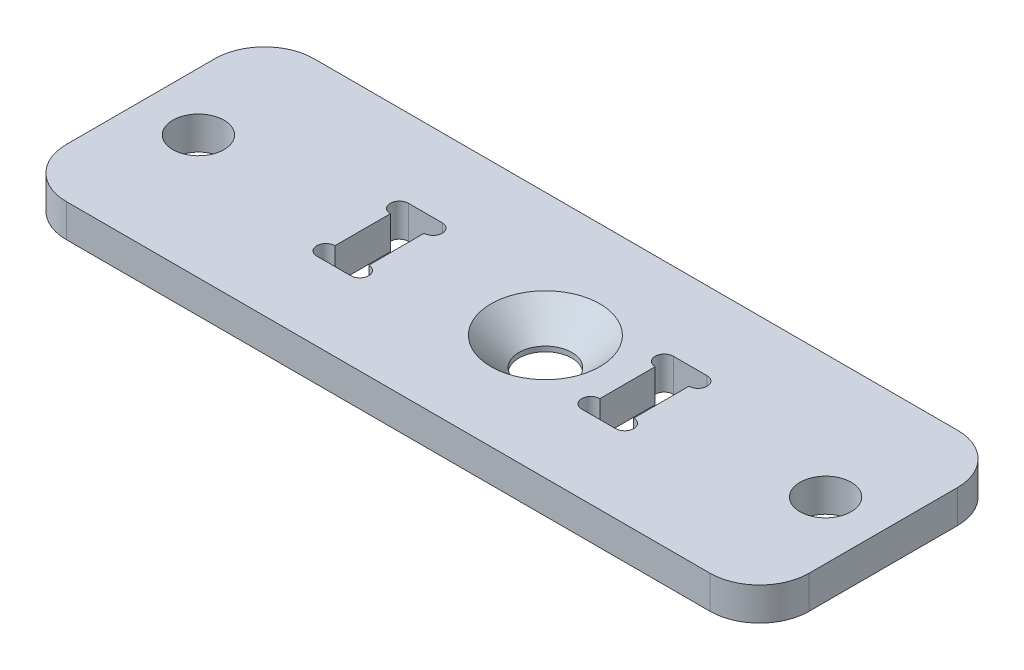
SolidWorks part; units mm, degrees
material "Thornel Mat VMA"
ref_plane "前视基准面" through (0, 0, 0) normal (0, 0, 1) x (1, 0, 0)
ref_plane "上视基准面" through (0, 0, 0) normal (0, 1, 0) x (1, 0, 0)
ref_plane "右视基准面" through (0, 0, 0) normal (1, 0, 0) x (0, 0, -1)
other "Configuration Table"
sketch "草图1" plane through (0, 0, 0) normal (0, 1, 0) x (1, 0, 0)
  line L0 (0, 0) -> (37.6995, 0) construction
  line L1 (-22.5, 7.5) -> (22.5, 7.5)
  line L2 (-22.5, 7.5) -> (-22.5, -7.5)
  line L3 (-22.5, -7.5) -> (22.5, -7.5)
  line L4 (22.5, 7.5) -> (22.5, -7.5)
  line L5 (-22.5, 7.5) -> (22.5, -7.5) construction
  line L6 (-22.5, -7.5) -> (22.5, 7.5) construction
  line L7 (0, 0) -> (0, 17.3296) construction
  line L8 (8.025, 0) -> (8.025, 5.6188) construction
  line L9 (7, 2.775) -> (9.05, 2.775)
  line L10 (7, 2.775) -> (7, -2.775)
  line L11 (7, -2.775) -> (9.05, -2.775)
  line L12 (9.05, 2.775) -> (9.05, -2.775)
  line L13 (7, 2.775) -> (9.05, -2.775) construction
  line L14 (7, -2.775) -> (9.05, 2.775) construction
  line L15 (-7, -2.775) -> (-9.05, 2.775) construction
  line L16 (-7, 2.775) -> (-9.05, -2.775) construction
  line L21 (-9.05, 2.775) -> (-9.05, -2.775)
  line L22 (-7, -2.775) -> (-9.05, -2.775)
  line L23 (-7, 2.775) -> (-7, -2.775)
  line L24 (-7, 2.775) -> (-9.05, 2.775)
  circle A0 centre (19, 0) radius 1.55
  circle A1 centre (-19, 0) radius 1.55
  circle A6 centre (2.025, 0) radius 1.55
  circle A11 centre (9.05, 2.225) radius 0.55
  circle A12 centre (7, 2.225) radius 0.55
  circle A13 centre (9.05, -2.225) radius 0.55
  circle A14 centre (7, -2.225) radius 0.55
  circle A15 centre (-7, -2.225) radius 0.55
  circle A16 centre (-9.05, -2.225) radius 0.55
  circle A17 centre (-7, 2.225) radius 0.55
  circle A18 centre (-9.05, 2.225) radius 0.55
  point P0 (0, 0)
  point P13 (8.025, 0)
  point P42 (-8.025, 0)
  dimension "D1" = 3.1
  dimension "D2" = 38
  dimension "D6" = 1.1
  dimension "D7" = 45
  dimension "D8" = 6
  dimension "D3" = 7
  dimension "D4" = 2.05
  dimension "D5" = 5.55
  dimension "D9" = 15
extrude "凸台-拉伸1" add sketch "草图1" along normal blind 2
fillet "圆角1" radius 3 4 edges at (22.5, 1, 7.5) (-22.5, 1, 7.5) (22.5, 1, -7.5) (-22.5, 1, -7.5)
hole_wizard "M3 十字槽半沉头木螺钉的锥形沉头孔1" positions "草图4" profile "草图3" countersink size "M3" standard "GB"
sketch "草图4" plane through (0, 2, 0) normal (0, 1, 0) x (1, 0, 0)
  point P0 (2.025, 0)
sketch "草图3" plane through (2.025, 2, 0) normal (1, 0, 0) x (0, 0, 1)
  line L0 (0, 0) -> (0, 8.4614)
  line L1 (0, 8.4614) -> (1.6, 7.5)
  line L2 (1.6, 7.5) -> (1.6, 1.7)
  line L3 (1.6, 1.7) -> (3.3, 0)
  line L5 (3.3, 0) -> (0, 0)
  line L6 (-1.6, 1.7) -> (-3.3, 0) construction
  line L10 (0, 8.4614) -> (-1.6, 7.5) construction
  line L11 (0, -6.35) -> (0, 107.95) construction
  dimension "孔直径" = 3.2
  dimension "孔深度" = 7.5
  dimension "近端锥形沉头孔直径" = 6.6
  dimension "近端锥形沉头孔角度" = 90
  dimension "导头角度" = 118
